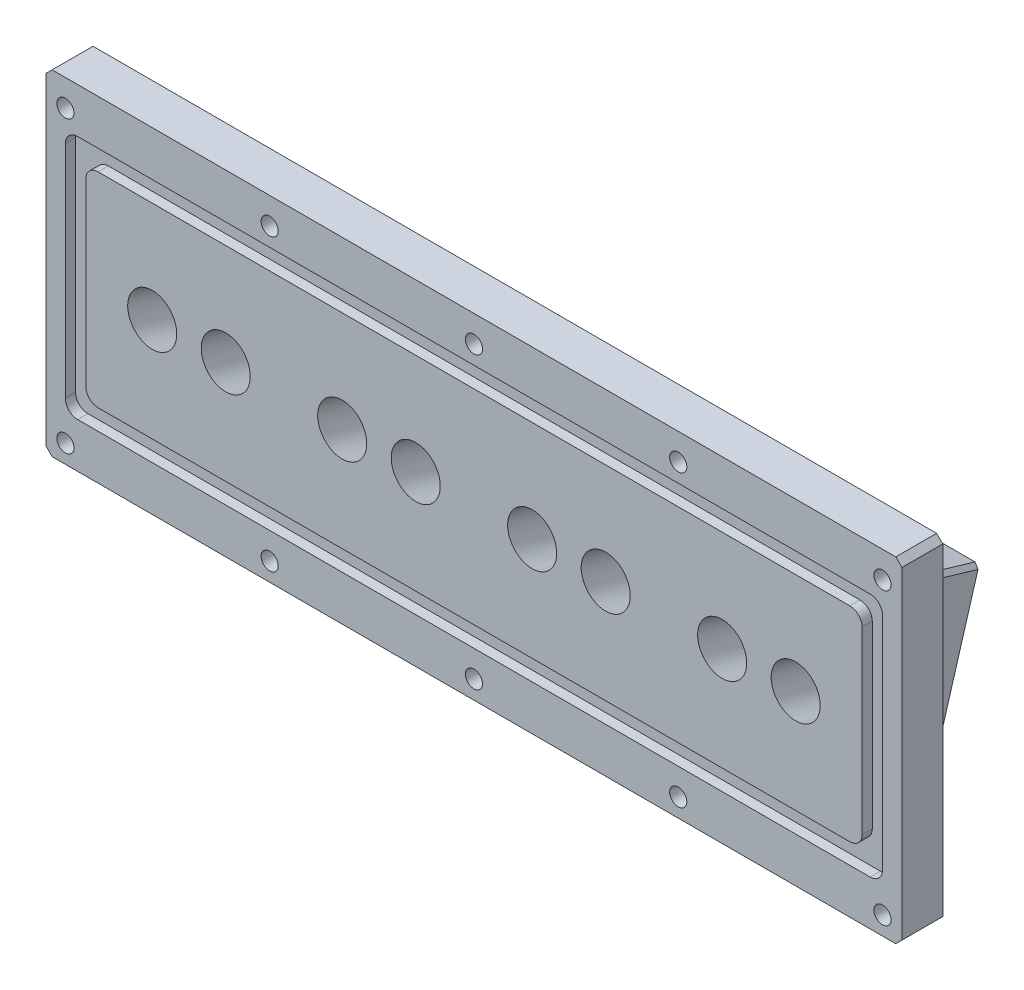
SolidWorks part; units mm, degrees
material "Q235-A"
ref_plane "Front Plane" through (0, 0, 0) normal (0, 0, 1) x (1, 0, 0)
ref_plane "Top Plane" through (0, 0, 0) normal (0, 1, 0) x (1, 0, 0)
ref_plane "Right Plane" through (0, 0, 0) normal (1, 0, 0) x (0, 0, -1)
sketch "Sketch1" plane through (0, 0, 0) normal (0, 0, 1) x (1, 0, 0)
  line L1 (-209.5, -82) -> (209.5, -82)
  line L2 (-209.5, -82) -> (-209.5, 82)
  line L3 (-209.5, 82) -> (209.5, 82)
  line L4 (209.5, -82) -> (209.5, 82)
  line L5 (-209.5, -82) -> (209.5, 82) construction
  line L6 (-209.5, 82) -> (209.5, -82) construction
  point P0 (0, 0)
  dimension "D1" = 419
  dimension "D2" = 164
extrude "Boss-Extrude1" add sketch "Sketch1" along normal blind 20
sketch "Sketch2" plane through (0, 0, 20) normal (0, 0, 1) x (1, 0, 0)
  line L1 (-200, -60) -> (200, -60)
  line L2 (-200, -60) -> (-200, 60)
  line L3 (-200, 60) -> (200, 60)
  line L4 (200, -60) -> (200, 60)
  line L5 (-200, -60) -> (200, 60) construction
  line L6 (-200, 60) -> (200, -60) construction
  line L7 (-190, -50) -> (190, -50)
  line L8 (-190, -50) -> (-190, 50)
  line L9 (-190, 50) -> (190, 50)
  line L10 (190, -50) -> (190, 50)
  line L11 (-190, -50) -> (190, 50) construction
  line L12 (-190, 50) -> (190, -50) construction
  point P0 (0, 0)
  point P6 (0, 0)
  dimension "D1" = 100
  dimension "D2" = 120
  dimension "D3" = 400
  dimension "D4" = 380
extrude "Cut-Extrude1" cut sketch "Sketch2" against normal blind 5
fillet "Fillet1" radius 6 8 edges at (190, 50, 17.5) (200, 60, 17.5) (190, -50, 17.5) (200, -60, 17.5) (-200, -60, 17.5) (-190, -50, 17.5) (-190, 50, 17.5) (-200, 60, 17.5)
chamfer "Chamfer1" distance 3 angle 45 4 edges at (-209.5, -82, 10) (-209.5, 82, 10) (209.5, -82, 10) (209.5, 82, 10)
sketch "Sketch3" plane through (0, 0, 0) normal (0, 0, -1) x (-1, 0, 0)
  line L0 (-206.5, 82) -> (206.5, 82) construction
  line L1 (-209.5, -79) -> (-209.5, 79) construction
  point P0 (-200, 69)
  point P8 (-100, 69)
  point P9 (0, 69)
  point P10 (100, 69)
  point P11 (200, 69)
  point P12 (-100, -73)
  point P13 (0, -73)
  point P14 (100, -73)
  point P15 (200, -73)
  point P16 (-200, -73)
  dimension "D1" = 13
  dimension "D2" = 9.5
  dimension "D3" = 5
  dimension "D4" = 2
hole_wizard "Hole1" positions "Sketch4" profile "Sketch5" legacy end condition through all
sketch "Sketch4" plane through (0, 0, 0) normal (0, 0, -1) x (-1, 0, 0)
  point P0 (-200, 69)
  point P3 (-200, -73)
  point P6 (-100, -73)
  point P9 (0, -73)
  point P12 (100, -73)
  point P15 (200, -73)
  point P18 (200, 69)
  point P21 (100, 69)
  point P24 (0, 69)
  point P27 (-100, 69)
sketch "Sketch5" plane through (200, 69, 0) normal (1, 0, 0) x (0, 1, 0)
  line L0 (0, 0) -> (0, 20)
  line L1 (0, 20) -> (4.2, 20)
  line L2 (4.2, 20) -> (4.2, 11)
  line L3 (4.2, 11) -> (7.5, 11)
  line L4 (7.5, 11) -> (7.5, 0)
  line L5 (7.5, 0) -> (0, 0)
  line L6 (0, 110) -> (0, -10) construction
  dimension "直径" = 8.4
  dimension "深度" = 20
  dimension "柱坑直径" = 15
  dimension "柱坑深度" = 11
ref_plane "Plane1" through (-189.5, 0, 0) normal (-1, 0, 0) x (0, 0, 1)
sketch "Sketch6" plane through (-189.5, 0, 0) normal (-1, 0, 0) x (0, 0, 1)
  line L0 (0, 52.67) -> (-37.82, 41.4702)
  line L1 (0, 79) -> (0, -79) construction
  line L2 (-37.82, 41.4702) -> (-6.5783, -64)
  line L3 (-6.5783, -64) -> (0, -64)
  line L4 (0, -64) -> (0, 52.67)
  line L5 (20, -82) -> (0, -82) construction
  line L6 (20, 79) -> (20, -79) construction
  dimension "D1" = 116.67
  dimension "D2" = 18
  dimension "D3" = 57.82
  dimension "D4" = 110
  dimension "D5" = 16.5
  dimension "D6" = 6.5783
extrude "Boss-Extrude2" add sketch "Sketch6" against normal blind 379
chamfer "Chamfer2" distance 2 angle 45 4 edges at (189.5, -64, -3.2892) (189.5, 47.0701, -18.91) (-189.5, -64, -3.2892) (-189.5, 47.0701, -18.91)
sketch "Sketch7" plane through (0, -6.9539, -23.4761) normal (0, -0.284, -0.9588) x (-1, 0, 0)
  line L0 (-187.5, 50.501) -> (187.5, 50.501) construction
  line L1 (209.5, 75.7468) -> (209.5, -75.7468) construction
  line L2 (16.5, -50.199) -> (16.5, 39.801)
  line L3 (109.5, -50.199) -> (169.5, -50.199)
  line L4 (109.5, -50.199) -> (109.5, 39.801)
  line L5 (109.5, 39.801) -> (169.5, 39.801)
  line L6 (169.5, -50.199) -> (169.5, 39.801)
  line L7 (109.5, -50.199) -> (169.5, 39.801) construction
  line L8 (109.5, 39.801) -> (169.5, -50.199) construction
  line L9 (16.5, -50.199) -> (76.5, -50.199)
  line L10 (76.5, -50.199) -> (76.5, 39.801)
  line L11 (16.5, 39.801) -> (76.5, 39.801)
  line L12 (-76.5, -50.199) -> (-76.5, 39.801)
  line L13 (-76.5, -50.199) -> (-16.5, -50.199)
  line L14 (-16.5, -50.199) -> (-16.5, 39.801)
  line L15 (-76.5, 39.801) -> (-16.5, 39.801)
  line L16 (-169.5, -50.199) -> (-169.5, 39.801)
  line L17 (-169.5, -50.199) -> (-109.5, -50.199)
  line L18 (-109.5, -50.199) -> (-109.5, 39.801)
  line L19 (-169.5, 39.801) -> (-109.5, 39.801)
  point P0 (157.5, -5.199)
  point P3 (121.5, -5.199)
  point P6 (139.5, -5.199)
  point P8 (64.5, -5.199)
  point P9 (28.5, -5.199)
  point P10 (-28.5, -5.199)
  point P11 (-64.5, -5.199)
  point P12 (-121.5, -5.199)
  point P13 (-157.5, -5.199)
  dimension "D1" = 55.7
  dimension "D2" = 52
  dimension "D3" = 36
  dimension "D5" = 40
  dimension "D6" = 60
  dimension "D7" = 90
  dimension "D8" = 10.7
  dimension "D4" = 4
  dimension "D9" = 4
hole_wizard "Hole2" positions "Sketch8" profile "Sketch9" legacy end condition through all
sketch "Sketch8" plane through (0, -6.9539, -23.4761) normal (0, -0.284, -0.9588) x (-1, 0, 0)
  point P0 (157.5, -5.199)
  point P3 (121.5, -5.199)
  point P6 (64.5, -5.199)
  point P9 (28.5, -5.199)
  point P12 (-28.5, -5.199)
  point P15 (-64.5, -5.199)
  point P18 (-121.5, -5.199)
  point P21 (-157.5, -5.199)
sketch "Sketch9" plane through (-157.5, -11.9388, -21.9995) normal (1, 0, 0) x (0, 0.9588, -0.284)
  line L0 (0, 0) -> (0, 66.9501)
  line L1 (0, 66.9501) -> (12, 66.9501)
  line L2 (12, 66.9501) -> (12, 0)
  line L3 (12, 0) -> (0, 0)
  line L4 (0, 110) -> (0, -10) construction
  dimension "直径" = 24
  dimension "深度" = 66.9501
hole_wizard "M6 Tapped Hole1" positions "Sketch10" profile "Sketch11" tap size "M6" standard "GB"
sketch "Sketch10" plane through (0, -6.9539, -23.4761) normal (0, -0.284, -0.9588) x (-1, 0, 0)
  point P0 (-169.5, 39.801)
  point P3 (-109.5, 39.801)
  point P6 (-76.5, 39.801)
  point P9 (-16.5, 39.801)
  point P12 (16.5, 39.801)
  point P15 (76.5, 39.801)
  point P18 (109.5, 39.801)
  point P21 (169.5, 39.801)
  point P24 (169.5, -50.199)
  point P27 (109.5, -50.199)
  point P30 (76.5, -50.199)
  point P33 (16.5, -50.199)
  point P36 (-16.5, -50.199)
  point P39 (-76.5, -50.199)
  point P42 (-109.5, -50.199)
  point P45 (-169.5, -50.199)
sketch "Sketch11" plane through (169.5, 31.2081, -34.7802) normal (1, 0, 0) x (0, 0.9588, -0.284)
  line L0 (0, 0) -> (0, 13.5022)
  line L1 (0, 13.5022) -> (2.5, 12)
  line L2 (2.5, 12) -> (2.5, 0)
  line L5 (2.5, 0) -> (0, 0)
  line L10 (0, 13.5022) -> (-2.5, 12) construction
  line L11 (0, -6.35) -> (0, 107.95) construction
  dimension "螺纹孔钻头直径" = 5
  dimension "螺纹孔钻头深度" = 12
  dimension "导头角度" = 118
cosmetic thread "Cosmetic Thread1" parameters "D1"=12, "D2"=6
cosmetic thread "Cosmetic Thread2" parameters "D1"=12, "D2"=6
cosmetic thread "Cosmetic Thread3" parameters "D1"=12, "D2"=6
cosmetic thread "Cosmetic Thread4" parameters "D1"=12, "D2"=6
cosmetic thread "Cosmetic Thread5" parameters "D1"=12, "D2"=6
cosmetic thread "Cosmetic Thread6" parameters "D1"=12, "D2"=6
cosmetic thread "Cosmetic Thread7" parameters "D1"=12, "D2"=6
cosmetic thread "Cosmetic Thread8" parameters "D1"=12, "D2"=6
cosmetic thread "Cosmetic Thread9" parameters "D1"=12, "D2"=6
cosmetic thread "Cosmetic Thread10" parameters "D1"=12, "D2"=6
cosmetic thread "Cosmetic Thread11" parameters "D1"=12, "D2"=6
cosmetic thread "Cosmetic Thread12" parameters "D1"=12, "D2"=6
cosmetic thread "Cosmetic Thread13" parameters "D1"=12, "D2"=6
cosmetic thread "Cosmetic Thread14" parameters "D1"=12, "D2"=6
cosmetic thread "Cosmetic Thread15" parameters "D1"=12, "D2"=6
cosmetic thread "Cosmetic Thread16" parameters "D1"=12, "D2"=6
sketch "Sketch12" plane through (0, -6.9539, -23.4761) normal (0, -0.284, -0.9588) x (-1, 0, 0)
  line L0 (209.5, 75.7468) -> (209.5, -75.7468) construction
  line L1 (-179.5, 33.8039) -> (179.5, 33.8039)
  line L2 (-179.5, 33.8039) -> (-179.5, -44.1961)
  line L3 (-179.5, -44.1961) -> (179.5, -44.1961)
  line L4 (179.5, 33.8039) -> (179.5, -44.1961)
  line L5 (-187.5, 50.5039) -> (187.5, 50.5039) construction
  dimension "D1" = 359
  dimension "D2" = 30
  dimension "D3" = 78
  dimension "D4" = 16.7
extrude "Cut-Extrude2" cut sketch "Sketch12" against normal blind 15
fillet "Fillet2" radius 6 4 edges at (-179.5, -47.1999, -3.7326) (-179.5, 27.588, -25.8858) (179.5, -47.1999, -3.7326) (179.5, 27.588, -25.8858)
